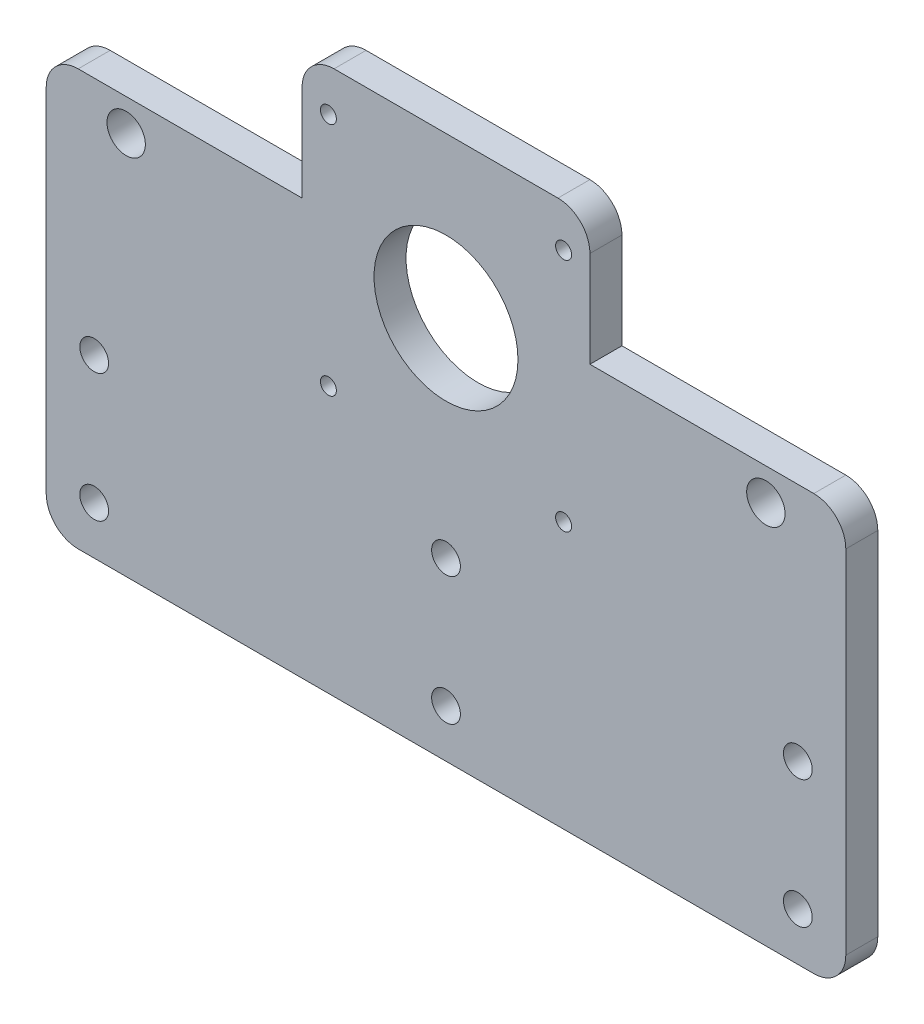
from build123d import *

# Parameters (mm, degrees)
SKETCH_1_W                = 250
SKETCH_1_H                = 170
EXTRUDE_1_DEPTH           = 5
SKETCH_2_W                = 80
SKETCH_2_H                = 40
CUT_EXTRUDE_1_DEPTH       = 10
HOLE_WIZARD_9_0_9_1_D     = 9
PATTERN_LINEAR_1_COUNT    = 3
PATTERN_LINEAR_1_PITCH    = 110
HOLE_WIZARD_12_0_12_1_D   = 12
SKETCH_7_R                = 22.5
CUT_EXTRUDE_2_DEPTH       = 10
HOLE_WIZARD_M6_1_D        = 5
PATTERN_LINEAR_3_COUNT    = 2
PATTERN_LINEAR_3_PITCH    = 73.54
PATTERN_LINEAR_4_COUNT    = 2
PATTERN_LINEAR_4_PITCH    = 73.54
PATTERN_LINEAR_4_COPY_1_D = 5
FILLET_1_R                = 10


with BuildPart() as part:
    # 草图1 → 凸台-拉伸1 (new, symmetric)
    with BuildSketch(Plane.XY):
        Rectangle(SKETCH_1_W, SKETCH_1_H)
    extrude(amount=EXTRUDE_1_DEPTH, both=True)

    # 草图2 → 切除-拉伸1 (cut)
    with BuildSketch(Plane.XY.offset(5)):
        with Locations((85, 65)):
            Rectangle(SKETCH_2_W, SKETCH_2_H)
    cut_extrude_1 = extrude(amount=-CUT_EXTRUDE_1_DEPTH, mode=Mode.SUBTRACT)

    # 镜向1: 切除-拉伸1 across plane
    add(cut_extrude_1.mirror(Plane(origin=(0, 0, 0), x_dir=(0, 0, 1), z_dir=(1, 0, 0))), mode=Mode.SUBTRACT)

    # Ø9.0 (9) 直径孔1 (through all)
    with Locations(Plane.XY.offset(5)):
        with Locations((-110, -70), (-110, -30)):
            hole_wizard_9_0_9_1 = Hole(HOLE_WIZARD_9_0_9_1_D / 2)

    # 阵列(线性)1: Ø9.0 (9) 直径孔1 ×3
    with Locations(*[(i * PATTERN_LINEAR_1_PITCH, 0, 0) for i in range(1, PATTERN_LINEAR_1_COUNT)]):
        add(hole_wizard_9_0_9_1, mode=Mode.SUBTRACT)

    # Ø12.0 (12) 直径孔1 (through all)
    with Locations(Plane.XY.offset(5)):
        with Locations((-100, 35), (100, 35)):
            Hole(HOLE_WIZARD_12_0_12_1_D / 2)

    # 草图7 → 切除-拉伸2 (cut)
    with BuildSketch(Plane.XY.offset(5)):
        with Locations((0, 35)):
            Circle(SKETCH_7_R)
    extrude(amount=-CUT_EXTRUDE_2_DEPTH, mode=Mode.SUBTRACT)

    # M6 螺纹孔1 (through all)
    with Locations(Plane.XY.offset(5)):
        with Locations((-36.77, 71.77)):
            hole_wizard_m6_1 = Hole(HOLE_WIZARD_M6_1_D / 2)

    # 阵列(线性)3: M6 螺纹孔1 ×2
    with Locations(*[(0, -i * PATTERN_LINEAR_3_PITCH, 0) for i in range(1, PATTERN_LINEAR_3_COUNT)]):
        add(hole_wizard_m6_1, mode=Mode.SUBTRACT)

    # 阵列(线性)4: M6 螺纹孔1 ×2
    with Locations(*[(i * PATTERN_LINEAR_4_PITCH, 0, 0) for i in range(1, PATTERN_LINEAR_4_COUNT)]):
        add(hole_wizard_m6_1, mode=Mode.SUBTRACT)

    # 阵列(线性)4 copy 1 (through all)
    with Locations(Plane(origin=(73.54, -73.54, 5), x_dir=(1, 0, 0), z_dir=(0, 0, 1))):
        with Locations((-36.77, 71.77)):
            Hole(PATTERN_LINEAR_4_COPY_1_D / 2)

    # 圆角1
    fillet_1_edges = [part.edges().sort_by_distance(p)[0] for p in [
        (125, 45, 0),
        (45, 85, 0),
        (-125, 45, 0),
        (-45, 85, 0),
        (125, -85, 0),
        (-125, -85, 0),
    ]]
    fillet(fillet_1_edges, radius=FILLET_1_R)


solid = part.part
